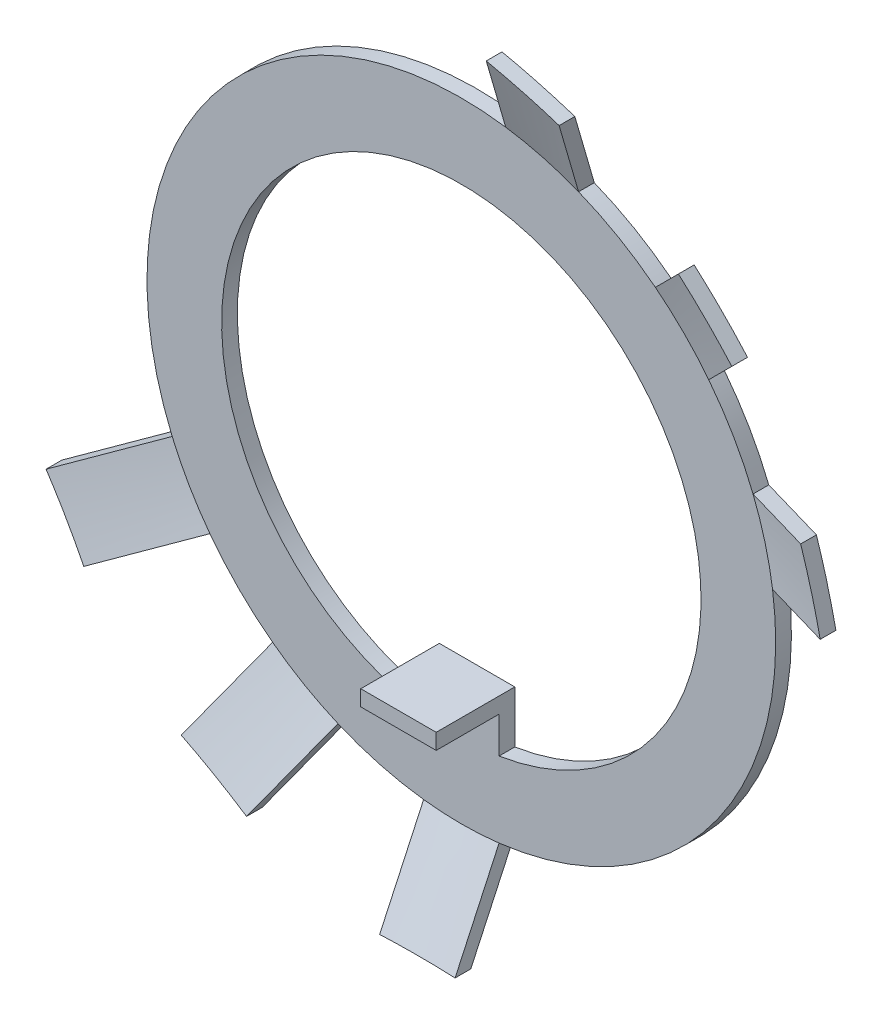
SolidWorks part; units mm, degrees
revolve "Base-Revolve" add sketch "Sketch2" angle 360 about L0
sketch "Sketch2" plane through (0, 0, 0) normal (1, 0, 0) x (0, 0, -1)
  line L0 (0, 0) -> (-1, 0) construction
  line L1 (-2.7978, 26) -> (0, 20)
  line L2 (0, 20) -> (0, 0)
  line L3 (-2.7978, 26) -> (-3.7978, 26)
  line L4 (-3.7978, 26) -> (-1, 20)
  line L5 (-1, 20) -> (-1, 0)
  line L6 (0, 0) -> (-1, 0)
extrude "Cut-Extrude2" cut sketch "Sketch3" along normal up to next flip side to cut
sketch "Sketch3" plane through (0, 0, 0) normal (0, 0, 1) x (1, 0, 0)
  line L0 (0, 0) -> (0, -25.889) construction
  line L1 (-2.4, -19.8555) -> (-2.4, -25.889)
  line L2 (-2.4, -25.889) -> (2.4, -25.889)
  line L3 (2.4, -19.8555) -> (2.4, -25.889)
  line L4 (2.4, -15.06) -> (2.4, -11.75)
  line L5 (2.4, -11.75) -> (-2.4, -11.75)
  line L6 (-2.4, -15.06) -> (-2.4, -11.75)
  line L7 (0, 0) -> (-12.9445, -22.4205) construction
  line L8 (0, 0) -> (-22.4205, -12.9445) construction
  line L9 (0, 0) -> (25.0068, 6.7006) construction
  line L10 (0, 0) -> (18.3063, 18.3063) construction
  line L11 (0, 0) -> (6.7006, 25.0068) construction
  line L12 (0, 0) -> (26, 0) construction
  line L13 (-15.023, -21.2205) -> (-10.866, -23.6205)
  line L14 (-10.866, -23.6205) -> (-7.8493, -18.3953)
  line L15 (-15.023, -21.2205) -> (-12.0062, -15.9953)
  line L16 (-15.9953, -12.0062) -> (-21.2205, -15.023)
  line L17 (-21.2205, -15.023) -> (-23.6205, -10.866)
  line L18 (-18.3953, -7.8493) -> (-23.6205, -10.866)
  line L19 (4.3823, 25.628) -> (9.0188, 24.3857)
  line L20 (9.0188, 24.3857) -> (7.4572, 18.5578)
  line L21 (4.3823, 25.628) -> (2.8208, 19.8001)
  line L22 (12.3429, 15.737) -> (16.6092, 20.0033)
  line L23 (16.6092, 20.0033) -> (20.0033, 16.6092)
  line L24 (15.737, 12.3429) -> (20.0033, 16.6092)
  line L25 (18.5578, 7.4572) -> (24.3857, 9.0188)
  line L26 (24.3857, 9.0188) -> (25.628, 4.3823)
  line L27 (19.8001, 2.8208) -> (25.628, 4.3823)
  arc A0 (2.4, -15.06) -> (-2.4, -15.06) centre (0, 0) ccw
  arc A1 (2.4, -19.8555) -> (19.8001, 2.8208) centre (0, 0) ccw
  circle A3 centre (0, 0) radius 26 construction
  arc A4 (-7.8493, -18.3953) -> (-2.4, -19.8555) centre (0, 0) ccw
  arc A5 (-15.9953, -12.0062) -> (-12.0062, -15.9953) centre (0, 0) ccw
  arc A6 (18.5578, 7.4572) -> (15.737, 12.3429) centre (0, 0) ccw
  arc A7 (12.3429, 15.737) -> (7.4572, 18.5578) centre (0, 0) ccw
  arc A8 (2.8208, 19.8001) -> (-18.3953, -7.8493) centre (0, 0) ccw
  point P14 (0, -11.75)
  point P25 (-12.9445, -22.4205)
  point P31 (-22.4205, -12.9445)
  point P35 (6.7006, 25.0068)
  point P40 (18.3063, 18.3063)
  point P45 (25.0068, 6.7006)
material "Q215"
ref_plane "Front Plane" through (0, 0, 0) normal (0, 0, 1) x (1, 0, 0)
ref_plane "Top Plane" through (0, 0, 0) normal (0, 1, 0) x (1, 0, 0)
ref_plane "Right Plane" through (0, 0, 0) normal (1, 0, 0) x (0, 0, -1)
sketch "Dimension Sketch" plane through (0, 0, 0) normal (0, 0, 1) x (1, 0, 0)
  line L0 (0, 0) -> (26, 0) construction
  line L1 (0, 0) -> (0, -26) construction
  circle A0 centre (0, 0) radius 26
  point P5 (5.8, 0)
  point P6 (21, 0)
  point P7 (4.8, 0)
  point P8 (-1, 0)
  point P10 (-4.5, 0)
  point P12 (0, 14)
sketch "Sketch4" plane through (0, 0, 0) normal (0, 0, 1) x (1, 0, 0)
  line L0 (2.4, -11.75) -> (2.4, -15.06) construction
  line L1 (-2.4, -11.75) -> (2.4, -11.75)
  line L2 (-2.4, -11.75) -> (-2.4, -12.75)
  line L3 (-2.4, -12.75) -> (2.4, -12.75)
  line L4 (2.4, -11.75) -> (2.4, -12.75)
extrude "Boss-Extrude1" add sketch "Sketch4" along normal blind 5
equation "\"D4@Sketch2\" = \"DD@Dimension Sketch\""
equation "\"D3@Sketch2\" = \"D1@Dimension Sketch\""
equation "\"D1@Sketch2\" = \"s@Dimension Sketch\""
equation "\"D4@Sketch3\" = \"a@Dimension Sketch\""
equation "\"D1@Sketch3\" = \"D1@Dimension Sketch\""
equation "\"D2@Sketch3\" = \"d@Dimension Sketch\""
equation "\"b@Sketch3\" = \"b@Dimension Sketch\""
equation "\"D1@Sketch4\" = \"s@Dimension Sketch\""
equation "\"D1@Boss-Extrude1\" = \"h@Dimension Sketch\""
equation "\"脚角度@Sketch3\" = sgn(101-\"d@Dimension Sketch\")*5+25"
equation "\"D7@Sketch3\" = sgn(\"d@Dimension Sketch\"-101)*2.5+17.5"
